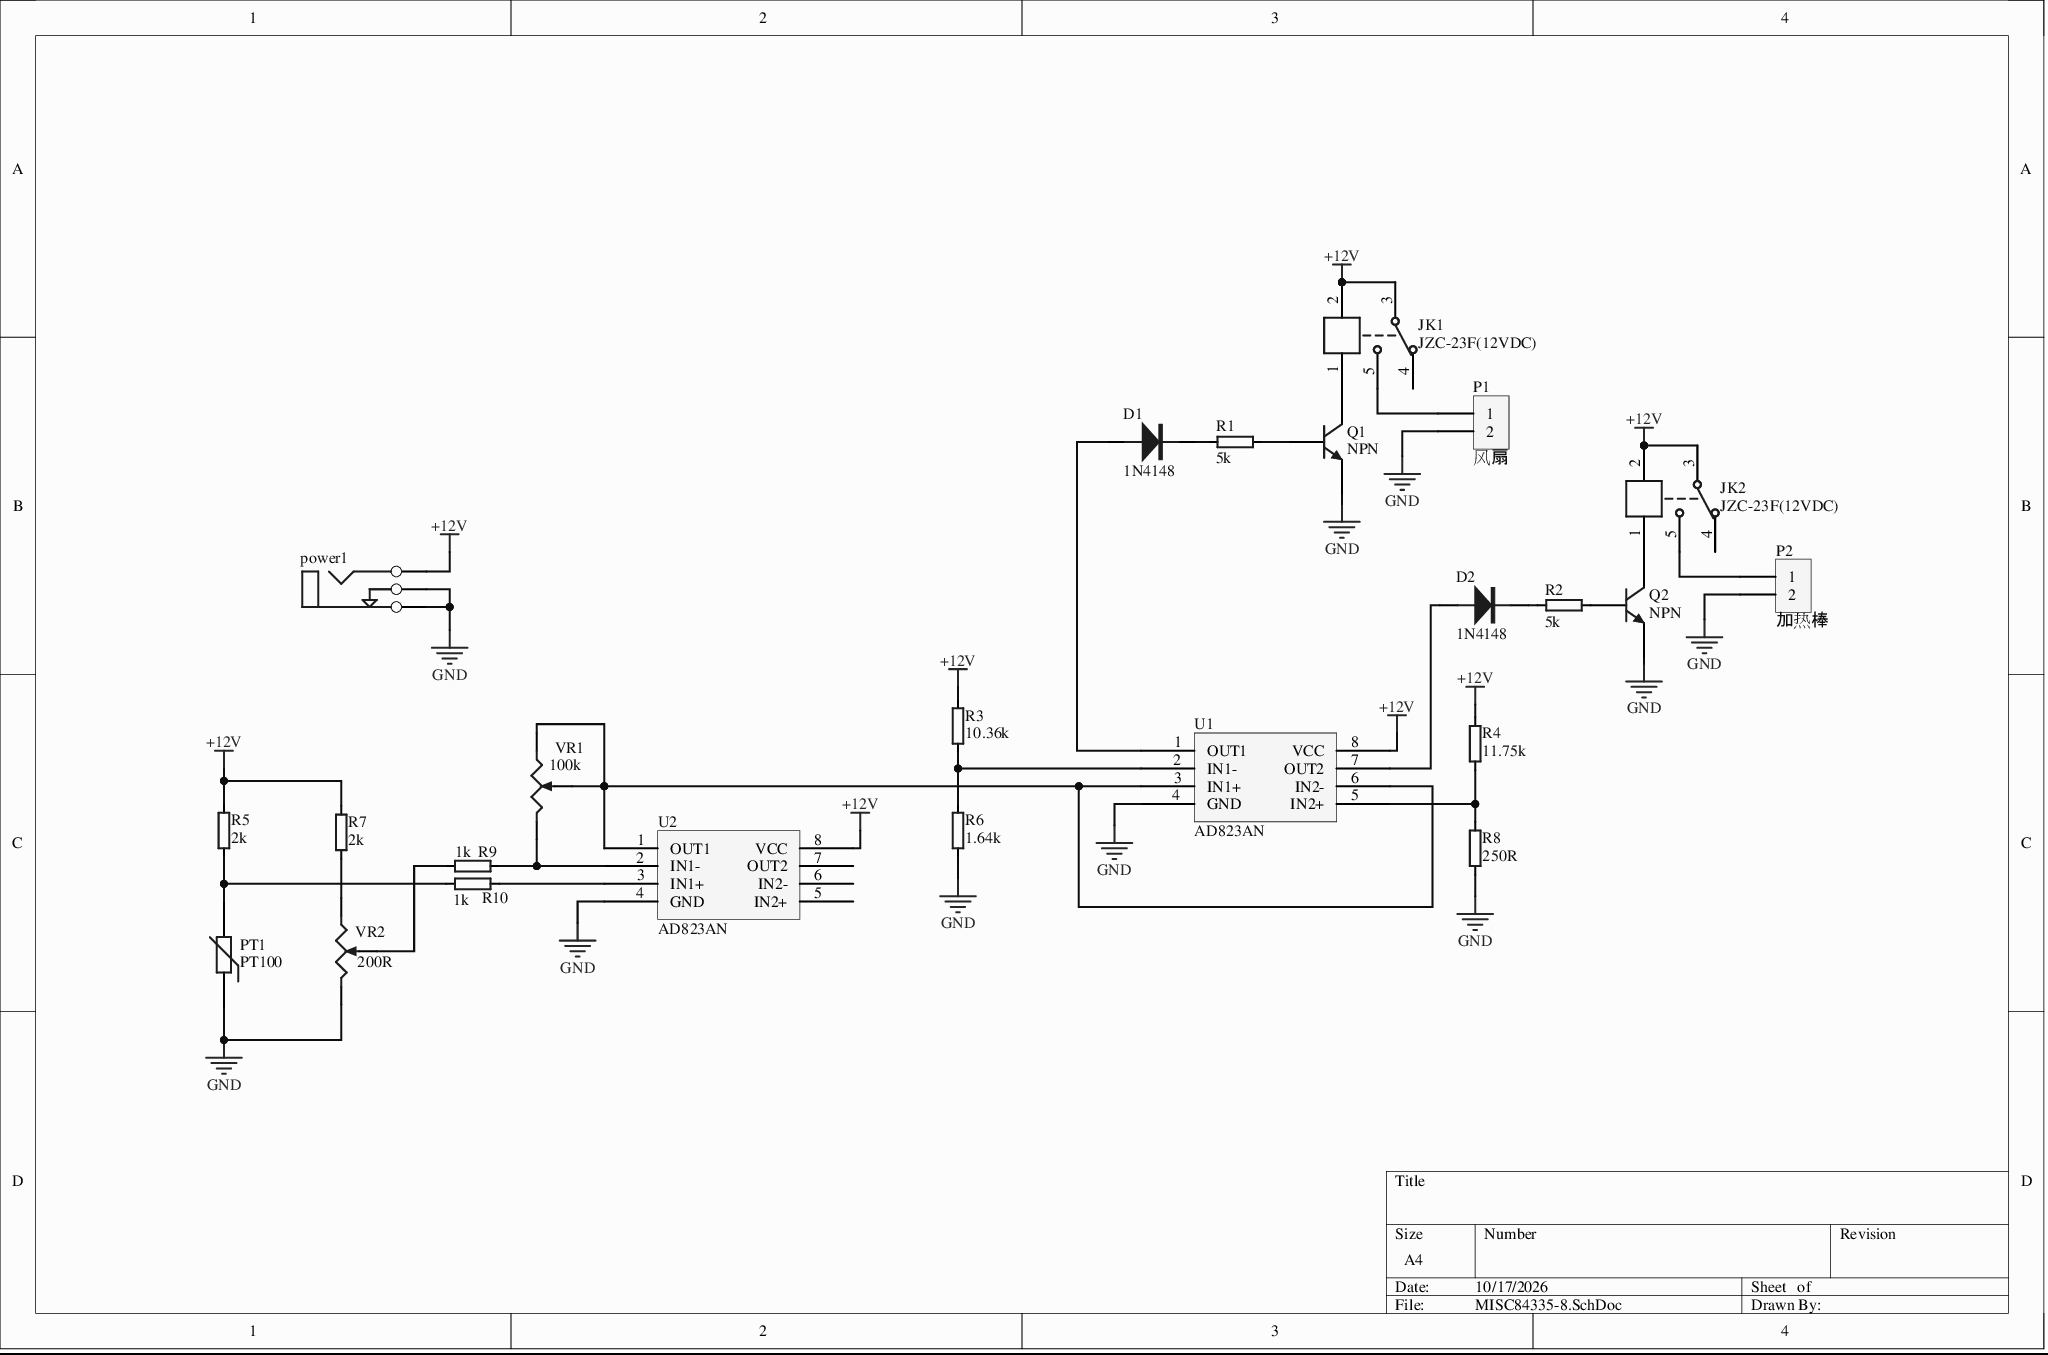
[diagram p0: MISC84335-8.SchDoc]
# Altium project MISC84335-2.PrjPcb
1 sheet, 24 parts. Net scope: global (net labels, ports and power ports of the same name join across sheets).
Board file: MISC84335.PcbDoc

## Sheet MISC84335-8.SchDoc
size A4

### Parts
D1  1N4148  [DO-35]
D2  1N4148  [DO-35]
JK1  JZC-23F(12VDC)  [JZC-23F(4123)]
JK2  JZC-23F(12VDC)  [JZC-23F(4123)]
P1  风扇  [HDR1X2]
P2  加热棒  [HDR1X2]
power1  (no value)  [DC-005]
PT1  PT100  [VDR 9D-4.5]
Q1  NPN  [TO-226-AA]
Q2  NPN  [TO-226-AA]
R1  5k  [RS 1/4W]
R2  5k  [RS 1/4W]
R3  10.36k  [RS 1/4W]
R4  11.75k  [RS 1/4W]
R5  2k  [RS 1/4W]
R6  1.64k  [RS 1/4W]
R7  2k  [RS 1/4W]
R8  250R  [RS 1/4W]
R9  1k  [RS 1/4W]
R10  1k  [RS 1/4W]
U1  AD823AN  [DIP-8]
U2  AD823AN  [DIP-8]
VR1  100k  [3296W]
VR2  200R  [3296W]

### Nets
+12V: JK1.2 JK1.3 JK2.2 JK2.3 power1.1(A) R3.2 R4.2 R5.2 R7.2 U1.8(VCC) U2.8(VCC)
GND: P1.2 P2.2 power1.2(B) power1.3(C) PT1.1 Q1.3(E) Q2.3(E) R6.1 R8.1 U1.4(GND) U2.4(GND) VR2.3(TOP)
NetD1_1: D1.1 U1.1(OUT1)
NetD1_2: D1.2 R1.2
NetD2_1: D2.1 U1.7(OUT2)
NetD2_2: D2.2 R2.2
NetJK1_1: JK1.1 Q1.1(C)
NetJK1_5: JK1.5 P1.1
NetJK2_1: JK2.1 Q2.1(C)
NetJK2_5: JK2.5 P2.1
NetPT1_2: PT1.2 R5.1 R10.2
NetQ1_2: Q1.2(B) R1.1
NetQ2_2: Q2.2(B) R2.1
NetR3_1: R3.1 R6.2 U1.2(IN1-)
NetR4_1: R4.1 R8.2 U1.5(IN2+)
NetR7_1: R7.1 VR2.1(BOT)
NetR9_1: R9.1 U2.2(IN1-) VR1.3(TOP)
NetR9_2: R9.2 VR2.2(TAP)
NetR10_1: R10.1 U2.3(IN1+)
NetU1_3: U1.3(IN1+) U1.6(IN2-) U2.1(OUT1) VR1.1(BOT) VR1.2(TAP)

Not connected (* = marked no-connect by the designer): JK1 4; JK2 4; U2 5(IN2+) 6(IN2-) 7(OUT2)

### Library data of the parts
D1 D2 = DIO: Diode
JK1 JK2 = JZC-23F(5VDC): 5V单路双控; BOM名称: BOM name text         5V relay
P1 P2 = CON2
power1 = power2
PT1 = Res Varistor
Q1 Q2 = NPN: NPN Bipolar Transistor; Published: 8-Jun-2000; LatestRevisionDate: 17-Jul-2002; LatestRevisionNote: Re-released for DXP Platform.; PackageReference: TO-226-AA; PackageDescription: TO, Flat Index; 3 In-Line, Axial Leads; Body Dia. 4.8mm; Leads 0.55 x 0.51 mm (max); Code_JEDEC: TO-226-AA; Publisher: Altium Limited
R1-R10 = RES
U1 U2 = LM358_2
VR1 VR2 = RES-V: Potentiometer